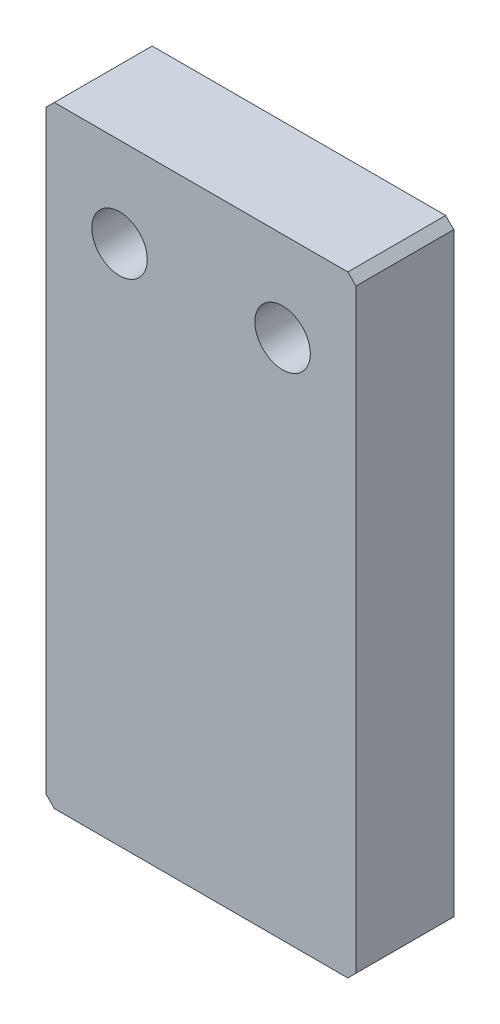
SolidWorks part; units mm, degrees
material "AL6061"
ref_plane "Front Plane" through (0, 0, 0) normal (0, 0, 1) x (1, 0, 0)
ref_plane "Top Plane" through (0, 0, 0) normal (0, 1, 0) x (1, 0, 0)
ref_plane "Right Plane" through (0, 0, 0) normal (1, 0, 0) x (0, 0, -1)
sketch "Sketch1" plane through (0, 0, 0) normal (0, 0, 1) x (1, 0, 0)
  line L1 (-19, 37.5) -> (19, 37.5)
  line L2 (-19, 37.5) -> (-19, -37.5)
  line L3 (-19, -37.5) -> (19, -37.5)
  line L4 (19, 37.5) -> (19, -37.5)
  line L5 (-19, 37.5) -> (19, -37.5) construction
  line L6 (-19, -37.5) -> (19, 37.5) construction
  point P0 (0, 0)
  dimension "D1" = 75
  dimension "D2" = 38
extrude "Boss-Extrude1" add sketch "Sketch1" along normal mid plane 12
hole_wizard "M8 Tapped Hole1" positions "Sketch3" profile "Sketch4" tap size "M8" standard "ISO" end condition through all
sketch "Sketch3" plane through (0, 0, 6) normal (0, 0, 1) x (1, 0, 0)
  line L0 (-19, -37.5) -> (19, -37.5) construction
  point P0 (-10, 26.5)
  dimension "D1" = 64
  dimension "D2" = 10
sketch "Sketch4" plane through (-10, 26.5, 6) normal (1, 0, 0) x (0, -1, 0)
  line L0 (0, 0) -> (0, 12)
  line L1 (0, 12) -> (3.4, 12)
  line L2 (3.4, 12) -> (3.4, 0)
  line L5 (3.4, 0) -> (0, 0)
  line L11 (0, -6.35) -> (0, 107.95) construction
  dimension "通孔螺纹孔钻头直径" = 6.8
  dimension "通孔螺纹孔钻头深度" = 12
cosmetic thread "Cosmetic thread 1" parameters "D2"=8
hole_wizard "M8 Tapped Hole2" positions "Sketch5" profile "Sketch6" tap size "M8" standard "ISO" end condition through all
sketch "Sketch5" plane through (0, 0, 6) normal (0, 0, 1) x (1, 0, 0)
  point P0 (10, 26.5)
  dimension "D1" = 10
sketch "Sketch6" plane through (10, 26.5, 6) normal (1, 0, 0) x (0, -1, 0)
  line L0 (0, 0) -> (0, 12)
  line L1 (0, 12) -> (3.4, 12)
  line L2 (3.4, 12) -> (3.4, 0)
  line L5 (3.4, 0) -> (0, 0)
  line L11 (0, -6.35) -> (0, 107.95) construction
  dimension "通孔螺纹孔钻头直径" = 6.8
  dimension "通孔螺纹孔钻头深度" = 12
cosmetic thread "Cosmetic thread 2" parameters "D2"=8
hole_wizard "M6 Tapped Hole1" positions "Sketch9" profile "Sketch10" tap size "M6" standard "ISO"
sketch "Sketch9" plane through (0, -37.5, 0) normal (0, -1, 0) x (-1, 0, 0)
  line L0 (0, 0) -> (0, -11.6211) construction
  point P0 (10, 0)
  point P2 (-10, 0)
  dimension "D1" = 20
cosmetic thread "Cosmetic thread 3" parameters "D1"=12, "D2"=6
cosmetic thread "Cosmetic thread 4" parameters "D1"=12, "D2"=6
sketch "Sketch10" plane through (-10, -37.5, 0) normal (1, 0, 0) x (0, 0, -1)
  line L0 (0, 0) -> (0, 12)
  line L1 (0, 12) -> (2.5, 12)
  line L2 (2.5, 12) -> (2.5, 0)
  line L5 (2.5, 0) -> (0, 0)
  line L10 (0, 12) -> (-2.5, 12) construction
  line L11 (0, -6.35) -> (0, 107.95) construction
  dimension "螺纹孔钻头直径" = 5
  dimension "螺纹孔钻头深度" = 12
  dimension "导头角度" = 180
chamfer "Chamfer1" distance 1 angle 45 4 edges at (19, 37.5, 0) (-19, 37.5, 0) (-19, -37.5, 0) (19, -37.5, 0)
